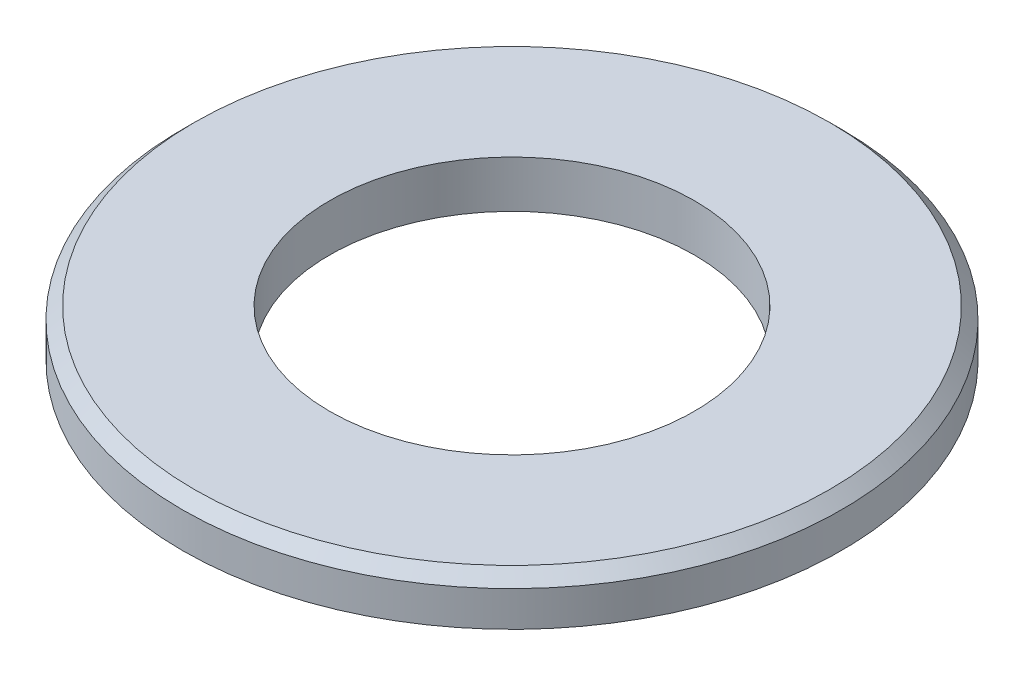
from build123d import *


with BuildPart() as part:
    # 草图1 → Revolve 481 (revolve)
    with BuildSketch(Plane.XY, mode=Mode.PRIVATE) as revolve_481_sk:
        Polygon((-27, 12.644507042), (-28, 11.644507042), (-28, 8.644507042), (-15.5, 8.644507042), (-15.5, 12.644507042), align=None)
    revolve(revolve_481_sk.sketch.rotate(Axis((0, 0, 0), (0, 1, 0)), 270), axis=Axis((0, 0, 0), (0, 1, 0)))


solid = part.part
